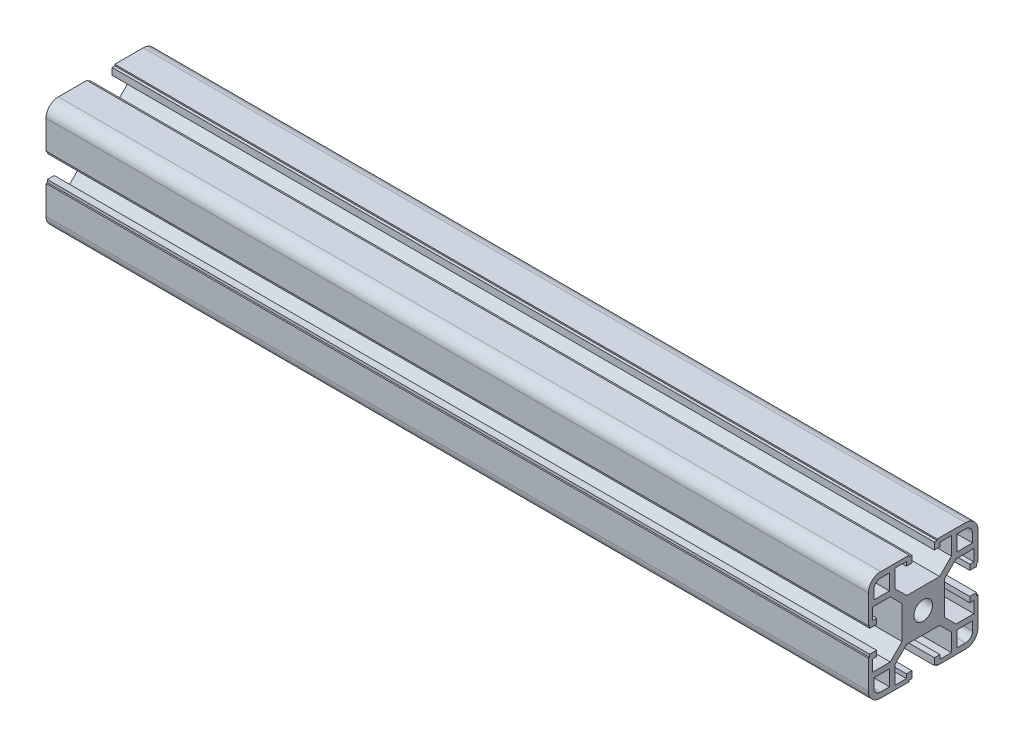
from build123d import *

# Parameters (mm, degrees)
SKETCH1_R                                = 3.4
ALUMINUM_PROFILE_40_X_40B_X_R4_5_1_DEPTH = 300


with BuildPart() as part:
    # Sketch1 → Aluminum profile 40 X 40B X R4.5(1) (new body)
    with BuildSketch(Plane.YZ):
        with BuildLine():
            Line((-5.1, 20), (-5.1, 19.5))
            Line((-5.1, 19.5), (-4.1, 19.5))
            Line((-4.1, 19.5), (-4.1, 17))
            Line((-4.1, 17), (-6.1, 17))
            Line((-6.1, 17), (-6.1, 18.5))
            Line((-6.1, 18.5), (-10.3, 18.5))
            Line((-10.3, 18.5), (-10.3, 12))
            Line((-10.3, 12), (-6, 7.7))
            Line((-6, 7.7), (6, 7.7))
            Line((6, 7.7), (10.3, 12))
            Line((10.3, 12), (10.3, 18.5))
            Line((10.3, 18.5), (6.1, 18.5))
            Line((6.1, 18.5), (6.1, 17))
            Line((6.1, 17), (4.1, 17))
            Line((4.1, 17), (4.1, 19.5))
            Line((4.1, 19.5), (5.1, 19.5))
            Line((5.1, 19.5), (5.1, 20))
            Line((5.1, 20), (15.5, 20))
            ThreePointArc((15.5, 20), (18.681980515, 18.681980515), (20, 15.5))
            Line((20, 15.5), (20, 5.1))
            Line((20, 5.1), (19.5, 5.1))
            Line((19.5, 5.1), (19.5, 4.1))
            Line((19.5, 4.1), (17, 4.1))
            Line((17, 4.1), (17, 6.1))
            Line((17, 6.1), (18.5, 6.1))
            Line((18.5, 6.1), (18.5, 10.3))
            Line((18.5, 10.3), (12, 10.3))
            Line((12, 10.3), (7.7, 6))
            Line((7.7, 6), (7.7, -6))
            Line((7.7, -6), (12, -10.3))
            Line((12, -10.3), (18.5, -10.3))
            Line((18.5, -10.3), (18.5, -6.1))
            Line((18.5, -6.1), (17, -6.1))
            Line((17, -6.1), (17, -4.1))
            Line((17, -4.1), (19.5, -4.1))
            Line((19.5, -4.1), (19.5, -5.1))
            Line((19.5, -5.1), (20, -5.1))
            Line((20, -5.1), (20, -15.5))
            ThreePointArc((20, -15.5), (18.681980515, -18.681980515), (15.5, -20))
            Line((15.5, -20), (5.1, -20))
            Line((5.1, -20), (5.1, -19.5))
            Line((5.1, -19.5), (4.1, -19.5))
            Line((4.1, -19.5), (4.1, -17))
            Line((4.1, -17), (6.1, -17))
            Line((6.1, -17), (6.1, -18.5))
            Line((6.1, -18.5), (10.3, -18.5))
            Line((10.3, -18.5), (10.3, -12))
            Line((10.3, -12), (6, -7.7))
            Line((6, -7.7), (-6, -7.7))
            Line((-6, -7.7), (-10.3, -12))
            Line((-10.3, -12), (-10.3, -18.5))
            Line((-10.3, -18.5), (-6.1, -18.5))
            Line((-6.1, -18.5), (-6.1, -17))
            Line((-6.1, -17), (-4.1, -17))
            Line((-4.1, -17), (-4.1, -19.5))
            Line((-4.1, -19.5), (-5.1, -19.5))
            Line((-5.1, -19.5), (-5.1, -20))
            Line((-5.1, -20), (-15.5, -20))
            ThreePointArc((-15.5, -20), (-18.681980515, -18.681980515), (-20, -15.5))
            Line((-20, -15.5), (-20, -5.1))
            Line((-20, -5.1), (-19.5, -5.1))
            Line((-19.5, -5.1), (-19.5, -4.1))
            Line((-19.5, -4.1), (-17, -4.1))
            Line((-17, -4.1), (-17, -6.1))
            Line((-17, -6.1), (-18.5, -6.1))
            Line((-18.5, -6.1), (-18.5, -10.3))
            Line((-18.5, -10.3), (-12, -10.3))
            Line((-12, -10.3), (-7.7, -6))
            Line((-7.7, -6), (-7.7, 6))
            Line((-7.7, 6), (-12, 10.3))
            Line((-12, 10.3), (-18.5, 10.3))
            Line((-18.5, 10.3), (-18.5, 6.1))
            Line((-18.5, 6.1), (-17, 6.1))
            Line((-17, 6.1), (-17, 4.1))
            Line((-17, 4.1), (-19.5, 4.1))
            Line((-19.5, 4.1), (-19.5, 5.1))
            Line((-19.5, 5.1), (-20, 5.1))
            Line((-20, 5.1), (-20, 15.5))
            ThreePointArc((-20, 15.5), (-18.681980515, 18.681980515), (-15.5, 20))
            Line((-15.5, 20), (-5.1, 20))
        make_face()
        Circle(SKETCH1_R, mode=Mode.SUBTRACT)
        with BuildLine():
            Line((12.3, 18), (15.5, 18))
            ThreePointArc((15.5, 18), (17.267766953, 17.267766953), (18, 15.5))
            Line((18, 15.5), (18, 12.3))
            Line((18, 12.3), (12.3, 12.3))
            Line((12.3, 12.3), (12.3, 18))
        make_face(mode=Mode.SUBTRACT)
        with BuildLine():
            Line((-15.5, 18), (-12.3, 18))
            Line((-12.3, 18), (-12.3, 12.3))
            Line((-12.3, 12.3), (-18, 12.3))
            Line((-18, 12.3), (-18, 15.5))
            ThreePointArc((-18, 15.5), (-17.267766953, 17.267766953), (-15.5, 18))
        make_face(mode=Mode.SUBTRACT)
        with BuildLine():
            Line((-18, -12.3), (-12.3, -12.3))
            Line((-12.3, -12.3), (-12.3, -18))
            Line((-12.3, -18), (-15.5, -18))
            ThreePointArc((-15.5, -18), (-17.267766953, -17.267766953), (-18, -15.5))
            Line((-18, -15.5), (-18, -12.3))
        make_face(mode=Mode.SUBTRACT)
        with BuildLine():
            Line((12.3, -12.3), (18, -12.3))
            Line((18, -12.3), (18, -15.5))
            ThreePointArc((18, -15.5), (17.267766953, -17.267766953), (15.5, -18))
            Line((15.5, -18), (12.3, -18))
            Line((12.3, -18), (12.3, -12.3))
        make_face(mode=Mode.SUBTRACT)
    extrude(amount=ALUMINUM_PROFILE_40_X_40B_X_R4_5_1_DEPTH)


solid = part.part
